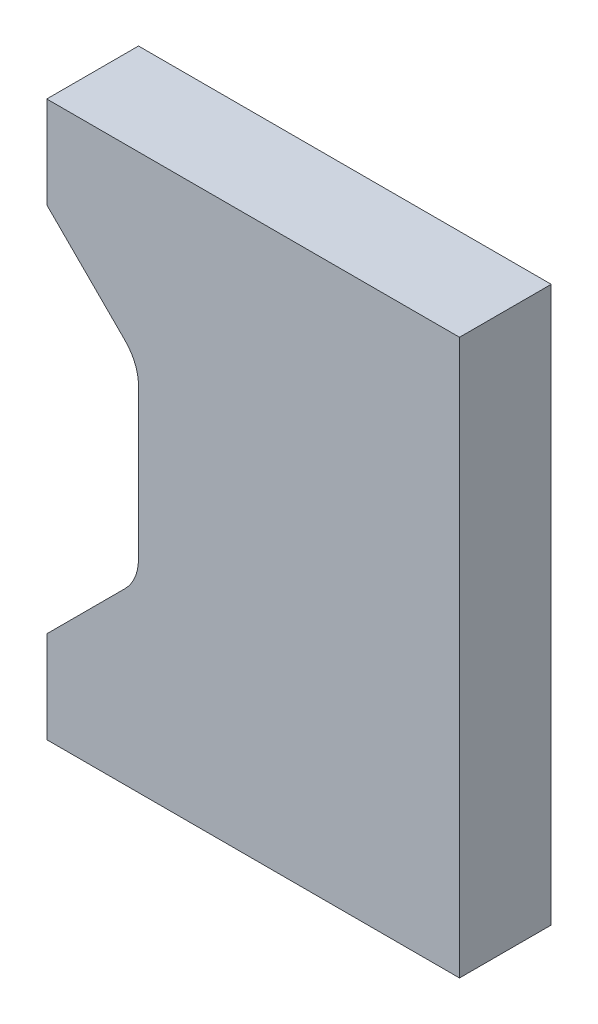
from build123d import *

# Parameters (mm, degrees)
BOSS_EXTRUDE1_DEPTH = 20


with BuildPart() as part:
    # Sketch1 → Boss-Extrude1 (new body)
    with BuildSketch(Plane.XY):
        with BuildLine():
            Line((0, 0), (90, 0))
            Line((90, 0), (90, -121))
            Line((90, -121), (0, -121))
            Line((0, -121), (0, -101))
            Line((0, -101), (17.071067812, -83.928932188))
            ThreePointArc((17.071067812, -83.928932188), (19.238795325, -80.6846987), (20, -76.857864376))
            Line((20, -76.857864376), (20, -44.142135624))
            ThreePointArc((20, -44.142135624), (19.238795325, -40.3153013), (17.071067812, -37.071067812))
            Line((17.071067812, -37.071067812), (0, -20))
            Line((0, -20), (0, 0))
        make_face()
    extrude(amount=BOSS_EXTRUDE1_DEPTH)


solid = part.part
